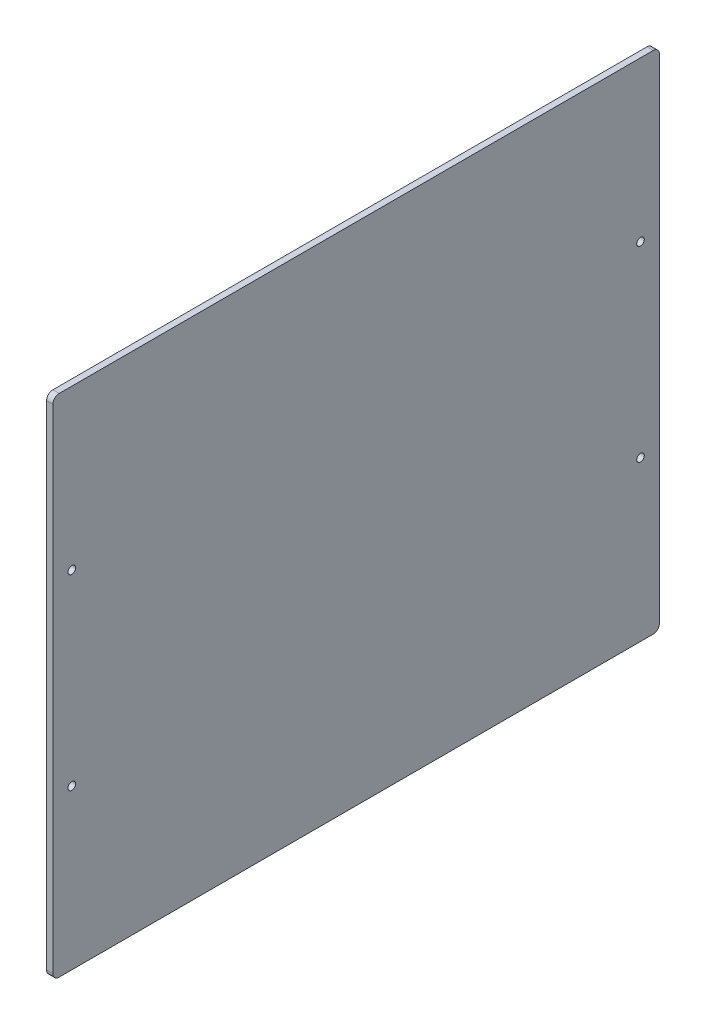
SolidWorks part; units mm, degrees
ref_plane "前视基准面" through (0, 0, 0) normal (0, 0, 1) x (1, 0, 0)
ref_plane "上视基准面" through (0, 0, 0) normal (0, 1, 0) x (1, 0, 0)
ref_plane "右视基准面" through (0, 0, 0) normal (1, 0, 0) x (0, 0, -1)
sketch "草图1" plane through (0, 0, 0) normal (1, 0, 0) x (0, 0, -1)
  line L0 (0, 200) -> (0, 0) construction
  line L1 (-240, 200) -> (240, 200)
  line L2 (-240, 200) -> (-240, -200)
  line L3 (-240, -200) -> (240, -200)
  line L4 (240, 200) -> (240, -200)
  line L5 (0, 0) -> (240, 0) construction
  dimension "D1" = 480
  dimension "D2" = 400
extrude "凸台-拉伸1" add sketch "草图1" along normal blind 5
sketch "草图2" plane through (5, 0, 0) normal (1, 0, 0) x (0, 0, -1)
  line L0 (0, 131.9543) -> (0, 0) construction
  line L1 (0, 0) -> (347.0268, 0) construction
  circle A0 centre (-225, 74) radius 3
  circle A1 centre (225, 74) radius 3
  circle A2 centre (-225, -74) radius 3
  circle A3 centre (225, -74) radius 3
  dimension "D1" = 6
  dimension "D2" = 450
  dimension "D3" = 148
extrude "切除-拉伸1" cut sketch "草图2" against normal through all
fillet "圆角1" radius 5 4 edges at (2.5, -200, 240) (2.5, -200, -240) (2.5, 200, -240) (2.5, 200, 240)
